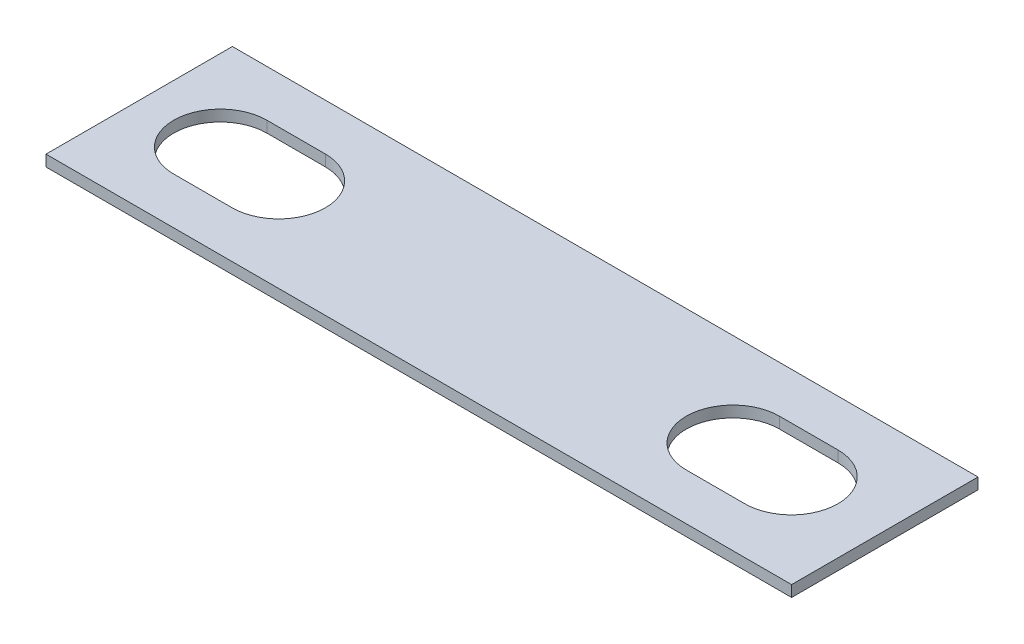
from build123d import *

# Parameters (mm, degrees)
SKETCH1_W           = 101.6
SKETCH1_H           = 25.4
BOSS_EXTRUDE1_DEPTH = 1.524


with BuildPart() as part:
    # Sketch1 → Boss-Extrude1 (new body)
    with BuildSketch(Plane(origin=(0, 0, 0), x_dir=(1, 0, 0), z_dir=(0, 1, 0))):
        with Locations((50.8, 12.7)):
            Rectangle(SKETCH1_W, SKETCH1_H)
        with BuildLine():
            Line((11.049, 19.05), (19.018813647, 19.05))
            ThreePointArc((19.018813647, 19.05), (25.368813647, 12.7), (19.018813647, 6.35))
            Line((19.018813647, 6.35), (11.049, 6.35))
            ThreePointArc((11.049, 6.35), (4.699, 12.7), (11.049, 19.05))
        make_face(mode=Mode.SUBTRACT)
        with BuildLine():
            Line((80.899, 19.05), (88.868813647, 19.05))
            ThreePointArc((88.868813647, 19.05), (95.218813647, 12.7), (88.868813647, 6.35))
            Line((88.868813647, 6.35), (80.899, 6.35))
            ThreePointArc((80.899, 6.35), (74.549, 12.7), (80.899, 19.05))
        make_face(mode=Mode.SUBTRACT)
    extrude(amount=BOSS_EXTRUDE1_DEPTH)


solid = part.part
